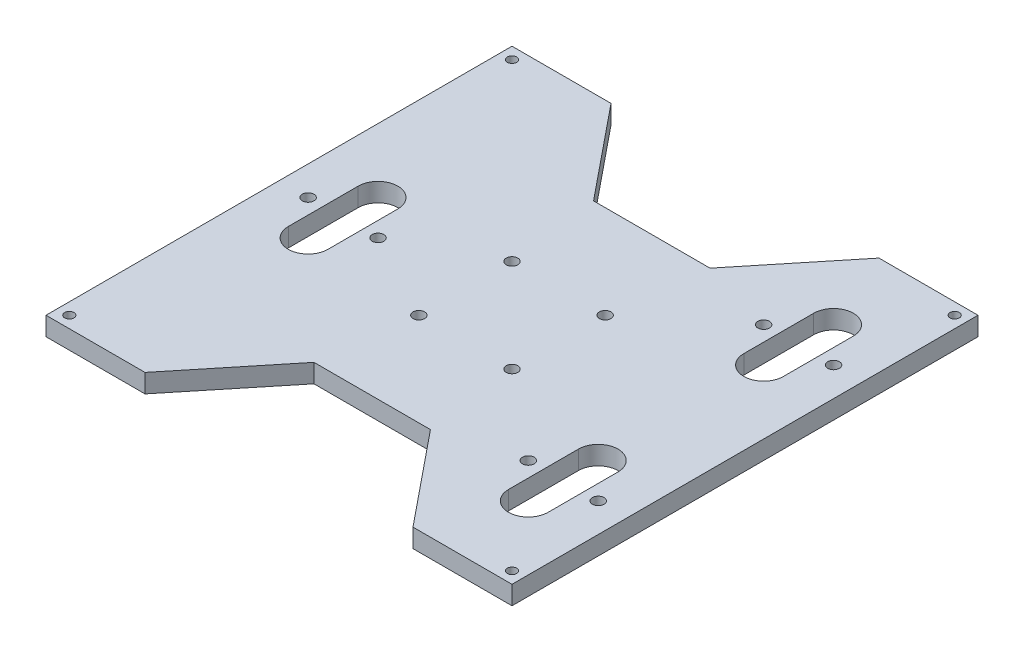
from build123d import *

# Parameters (mm, degrees)
SKETCH1_W           = 200
SKETCH1_H           = 200
SKETCH1_R           = 2
BOSS_EXTRUDE1_DEPTH = 8
SKETCH2_R           = 2.5
CUT_EXTRUDE1_DEPTH  = 283.955826941
CUT_EXTRUDE2_DEPTH  = 283.955826941


with BuildPart() as part:
    # Sketch1 → Boss-Extrude1 (new body)
    with BuildSketch(Plane(origin=(0, 0, 0), x_dir=(1, 0, 0), z_dir=(0, 1, 0))):
        with Locations((100, 100)):
            Rectangle(SKETCH1_W, SKETCH1_H)
        with Locations(Location((195, 195, 0), (0, 0, 270))):
            Circle(SKETCH1_R, mode=Mode.SUBTRACT)
        with Locations(Location((5, 195, 0), (0, 0, 270))):
            Circle(SKETCH1_R, mode=Mode.SUBTRACT)
        with Locations(Location((5, 5, 0), (0, 0, 270))):
            Circle(SKETCH1_R, mode=Mode.SUBTRACT)
        with Locations(Location((195, 5, 0), (0, 0, 270))):
            Circle(SKETCH1_R, mode=Mode.SUBTRACT)
    extrude(amount=BOSS_EXTRUDE1_DEPTH)

    # Sketch2 → Cut-Extrude1 (cut, through all)
    with BuildSketch(Plane.XZ):
        with Locations(Location((187.5, -49.5, 0), (0, 0, 270))):
            Circle(SKETCH2_R)
        with Locations(Location((157.5, -49.5, 0), (0, 0, 270))):
            Circle(SKETCH2_R)
        with Locations(Location((80, -120, 0), (0, 0, 270))):
            Circle(SKETCH2_R)
        with Locations(Location((80, -80, 0), (0, 0, 270))):
            Circle(SKETCH2_R)
        with Locations(Location((120, -80, 0), (0, 0, 270))):
            Circle(SKETCH2_R)
        with Locations(Location((120, -120, 0), (0, 0, 270))):
            Circle(SKETCH2_R)
        with Locations(Location((42.5, -100, 0), (0, 0, 270))):
            Circle(SKETCH2_R)
        with Locations(Location((12.5, -100, 0), (0, 0, 270))):
            Circle(SKETCH2_R)
        with Locations(Location((157.5, -150.5, 0), (0, 0, 270))):
            Circle(SKETCH2_R)
        with Locations(Location((187.5, -150.5, 0), (0, 0, 270))):
            Circle(SKETCH2_R)
    extrude(amount=-CUT_EXTRUDE1_DEPTH, mode=Mode.SUBTRACT)

    # Sketch3 → Cut-Extrude2 (cut, through all)
    with BuildSketch(Plane(origin=(0, 8, 0), x_dir=(1, 0, 0), z_dir=(0, 1, 0))):
        Polygon((42.5, 200), (75, 160), (125, 160), (157.5, 200), align=None)
        Polygon((42.5, 0), (157.5, 0), (125, 40), (75, 40), align=None)
        with BuildLine():
            Line((19, 85), (19, 115))
            ThreePointArc((19, 115), (27.5, 123.5), (36, 115))
            Line((36, 115), (36, 85))
            ThreePointArc((36, 85), (27.5, 76.5), (19, 85))
        make_face()
        with BuildLine():
            Line((181, 34.5), (181, 64.5))
            ThreePointArc((181, 64.5), (172.5, 73), (164, 64.5))
            Line((164, 64.5), (164, 34.5))
            ThreePointArc((164, 34.5), (172.5, 26), (181, 34.5))
        make_face()
        with BuildLine():
            Line((181, 165.5), (181, 135.5))
            ThreePointArc((181, 135.5), (172.5, 127), (164, 135.5))
            Line((164, 135.5), (164, 165.5))
            ThreePointArc((164, 165.5), (172.5, 174), (181, 165.5))
        make_face()
    extrude(amount=-CUT_EXTRUDE2_DEPTH, mode=Mode.SUBTRACT)


solid = part.part
